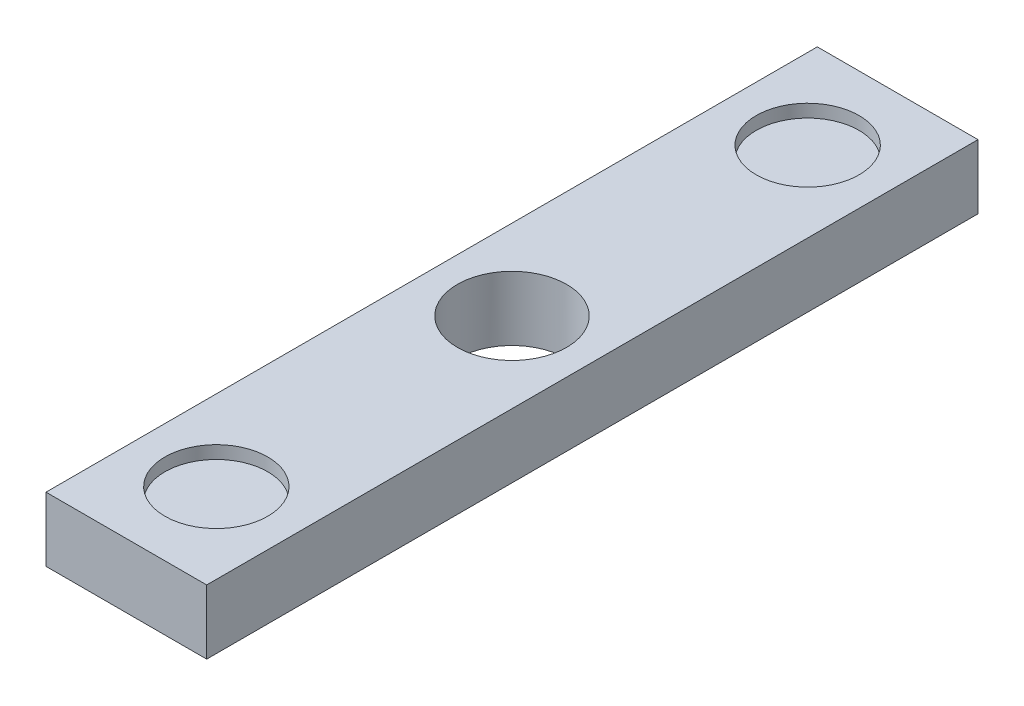
SolidWorks part; units mm, degrees
ref_plane "前视基准面" through (0, 0, 0) normal (0, 0, 1) x (1, 0, 0)
ref_plane "上视基准面" through (0, 0, 0) normal (0, 1, 0) x (1, 0, 0)
ref_plane "右视基准面" through (0, 0, 0) normal (1, 0, 0) x (0, 0, -1)
sketch "草图1" plane through (0, 0, 0) normal (0, 1, 0) x (1, 0, 0)
  line L1 (-12.5, -60) -> (12.5, -60)
  line L2 (-12.5, -60) -> (-12.5, 60)
  line L3 (-12.5, 60) -> (12.5, 60)
  line L4 (12.5, -60) -> (12.5, 60)
  line L5 (-12.5, -60) -> (12.5, 60) construction
  line L6 (-12.5, 60) -> (12.5, -60) construction
  point P0 (0, 0)
  dimension "D1" = 120
  dimension "D2" = 25
extrude "凸台-拉伸1" add sketch "草图1" along normal blind 10
sketch "草图2" plane through (0, 10, 0) normal (0, 1, 0) x (1, 0, 0)
  circle A0 centre (0, 46) radius 8
  circle A1 centre (0, -46) radius 8
extrude "切除-拉伸1" cut sketch "草图2" against normal blind 2
sketch "草图3" plane through (0, 10, 0) normal (0, 1, 0) x (1, 0, 0)
  circle A0 centre (0, 0) radius 8.5
  dimension "D1" = 17
extrude "切除-拉伸2" cut sketch "草图3" against normal up to next
equation "\"D3@草图2\"=\"D2@草图2\""
